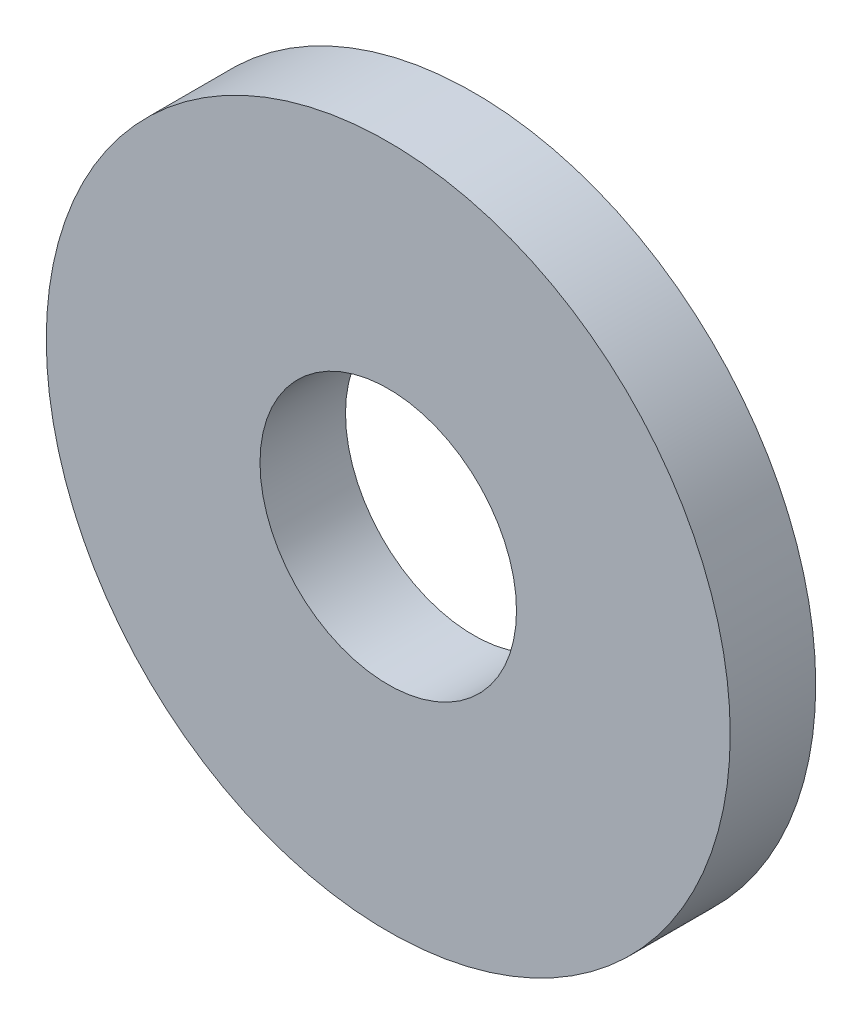
from build123d import *

# Parameters (mm, degrees)
SKETCH_1_R      = 8
SKETCH_1_R_2    = 3
EXTRUDE_1_DEPTH = 2


with BuildPart() as part:
    # 草图1 → 凸台-拉伸1 (new body)
    with BuildSketch(Plane.XY):
        Circle(SKETCH_1_R)
        Circle(SKETCH_1_R_2, mode=Mode.SUBTRACT)
    extrude(amount=EXTRUDE_1_DEPTH)


solid = part.part
